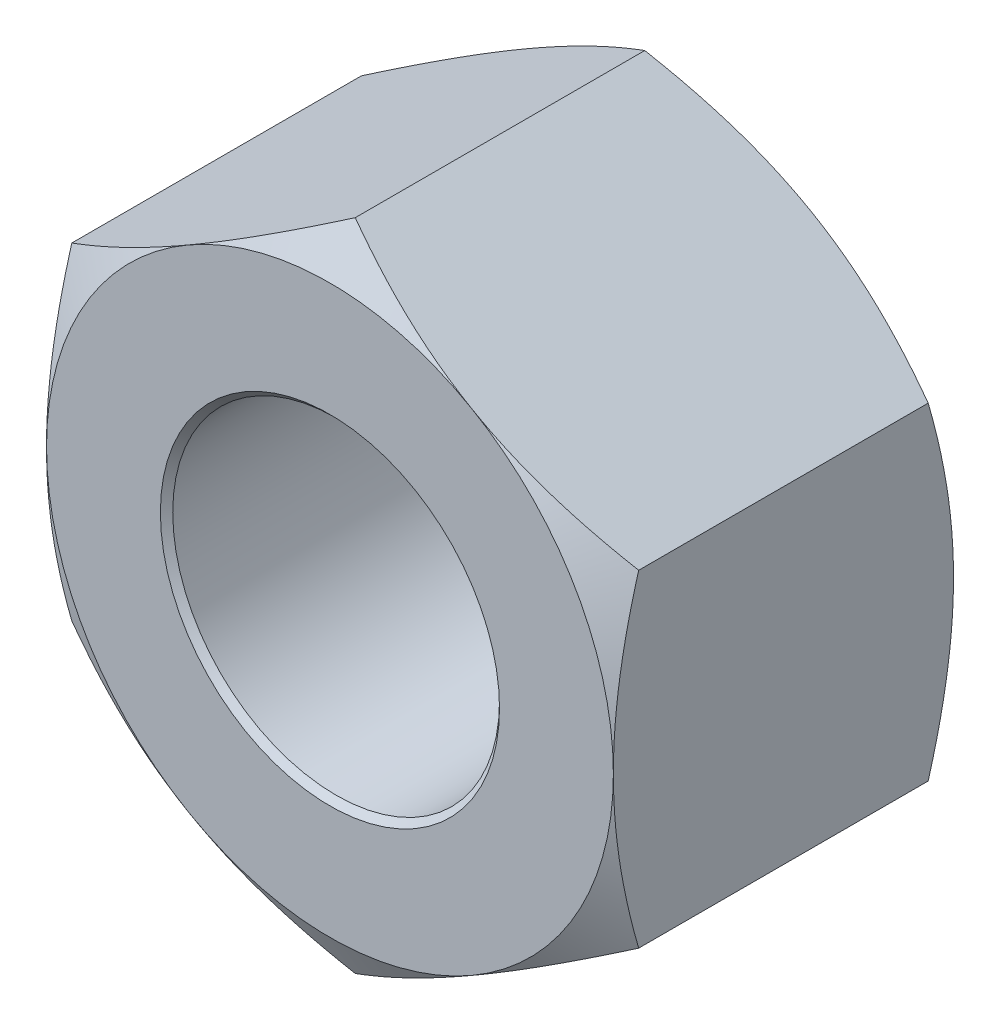
SolidWorks part; units mm, degrees
ref_plane "基准面1" through (0, 0, 0) normal (0, 0, 1) x (1, 0, 0)
ref_plane "基准面2" through (0, 0, 0) normal (0, 1, 0) x (1, 0, 0)
ref_plane "基准面3" through (0, 0, 0) normal (1, 0, 0) x (0, 0, -1)
sketch "尺寸草图" plane through (0, 0, 0) normal (0, 0, 1) x (1, 0, 0)
  line L0 (0, 0) -> (12, 0) construction
  line L1 (20.03, 0) -> (33.03, 0) construction
  line L2 (33.03, 0) -> (49.66, 0) construction
  line L3 (-11.4286, 0) -> (0, 0) construction
  point P0 (41.36, 0)
  point P3 (12, 0)
  point P4 (1.5, 0)
  point P5 (20.03, 0)
  point P6 (10.8, 0)
  point P8 (18, 0)
  dimension "D1" = 11.4286
  dimension "D" = 12
  dimension "P" = 1.5
  dimension "e(最小)" = 20.03
  dimension "m(最大)" = 10.8
  dimension "mw" = 8.3
  dimension "s(公称)" = 18
  dimension "da" = 13
  dimension "dw(最小)" = 16.63
sketch "草图1" plane through (0, 0, 0) normal (0, 0, 1) x (1, 0, 0)
  line L0 (-9, 0) -> (9, 0) construction
  line L1 (0, 10.3923) -> (0, -10.3923) construction
  line L3 (0, 10.3923) -> (-9, 5.1962)
  line L4 (-9, 5.1962) -> (-9, -5.1962)
  line L5 (-9, -5.1962) -> (0, -10.3923)
  line L6 (0, -10.3923) -> (9, -5.1962)
  line L7 (9, -5.1962) -> (9, 5.1962)
  line L8 (9, 5.1962) -> (0, 10.3923)
  circle A0 centre (0, 0) radius 9 construction
  circle A1 centre (0, 0) radius 5.1881
  point P2 (0, 9.6377)
  dimension "D1" = 18
  dimension "D" = 10.3763
  dimension "D2" = 20.03
extrude "基体-拉伸" add sketch "草图1" along normal blind 10.8
cosmetic thread "装饰螺纹线1" parameters "D2"=12
sketch "草图2" plane through (0, 0, 0) normal (0, 0, -1) x (-1, 0, 0)
  circle A0 centre (0, 0) radius 9
  circle A1 centre (0, 0) radius 5.1881 construction
  dimension "s" = 18
extrude "切除-拉伸1" cut sketch "草图2" against normal through all draft 60 flip side to cut
sketch "草图3" plane through (0, 0, 10.8) normal (0, 0, 1) x (1, 0, 0)
  circle A0 centre (0, 0) radius 9
  dimension "D1" = 18
extrude "切除-拉伸2" cut sketch "草图3" against normal through all draft 60 flip side to cut
chamfer "倒角1" distance 0.1964 angle 45 2 edges at (5.1881, 0, 0) (5.1881, 0, 10.8)
